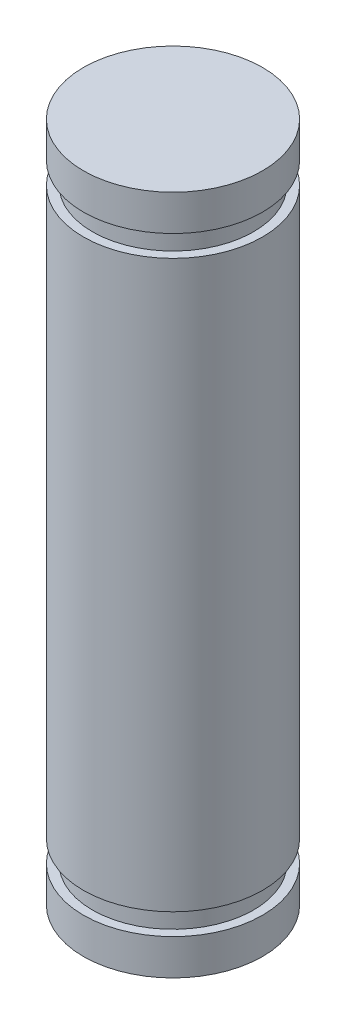
SolidWorks part; units mm, degrees
ref_plane "前视基准面" through (0, 0, 0) normal (0, 0, 1) x (1, 0, 0)
ref_plane "上视基准面" through (0, 0, 0) normal (0, 1, 0) x (1, 0, 0)
ref_plane "右视基准面" through (0, 0, 0) normal (1, 0, 0) x (0, 0, -1)
ref_plane "基准面4" through (0, 0, 0) normal (0, 0, -1) x (-1, 0, 0)
sketch "草图1" plane through (0, 0, 0) normal (0, 0, -1) x (-1, 0, 0)
  line L0 (-5, -19) -> (0, -19)
  line L1 (0, -19) -> (0, 19)
  line L2 (0, 19) -> (-5, 19)
  line L3 (-5, 19) -> (-5, 17)
  line L4 (-5, 17) -> (-4.5, 17)
  line L5 (-4.5, 17) -> (-4.5, 15.8)
  line L6 (-4.5, 15.8) -> (-5, 15.8)
  line L7 (-5, 15.8) -> (-5, -15.8)
  line L8 (-5, -15.8) -> (-4.5, -15.8)
  line L9 (-4.5, -15.8) -> (-4.5, -17)
  line L10 (-4.5, -17) -> (-5, -17)
  line L11 (-5, -17) -> (-5, -19)
  line L12 (0, -19) -> (0, 19) construction
revolve "旋转1" add sketch "草图1" angle 360 about L12
